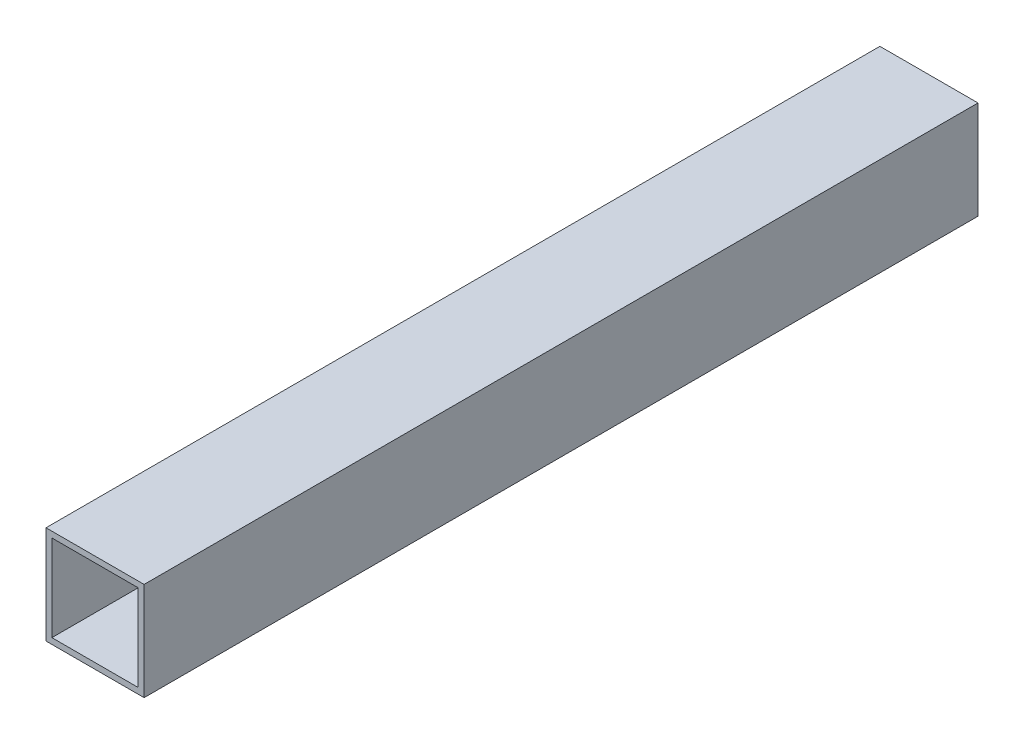
from build123d import *

# Parameters (mm, degrees)
SKETCH_1_W          = 50
SKETCH_1_H          = 50
SKETCH_1_W_2        = 44
SKETCH_1_H_2        = 44
EXTRUDE_1_DEPTH     = 400
SKETCH_2_W          = 50
SKETCH_2_H          = 50
SKETCH_2_W_2        = 44
SKETCH_2_H_2        = 44
CUT_EXTRUDE_1_DEPTH = 25
SKETCH_3_W          = 50
SKETCH_3_H          = 50
SKETCH_3_W_2        = 44
SKETCH_3_H_2        = 44
EXTRUDE_2_DEPTH     = 50


with BuildPart() as part:
    # 草图1 → 凸台-拉伸1 (new body)
    with BuildSketch(Plane.XY):
        with Locations((25, 25)):
            Rectangle(SKETCH_1_W, SKETCH_1_H)
        with Locations((25, 25)):
            Rectangle(SKETCH_1_W_2, SKETCH_1_H_2, mode=Mode.SUBTRACT)
    extrude(amount=EXTRUDE_1_DEPTH)

    # 草图2 → 切除-拉伸1 (cut)
    with BuildSketch(Plane(origin=(0, 0, 0), x_dir=(-1, 0, 0), z_dir=(0, 0, -1))):
        with Locations((-25, 25)):
            Rectangle(SKETCH_2_W, SKETCH_2_H)
        with Locations((-25, 25)):
            Rectangle(SKETCH_2_W_2, SKETCH_2_H_2, mode=Mode.SUBTRACT)
    extrude(amount=-CUT_EXTRUDE_1_DEPTH, mode=Mode.SUBTRACT)

    # 草图3 → 凸台-拉伸2 (add)
    with BuildSketch(Plane(origin=(0, 0, 25), x_dir=(-1, 0, 0), z_dir=(0, 0, -1))):
        with Locations((-25, 25)):
            Rectangle(SKETCH_3_W, SKETCH_3_H)
        with Locations((-25, 25)):
            Rectangle(SKETCH_3_W_2, SKETCH_3_H_2, mode=Mode.SUBTRACT)
    extrude(amount=EXTRUDE_2_DEPTH)


solid = part.part
